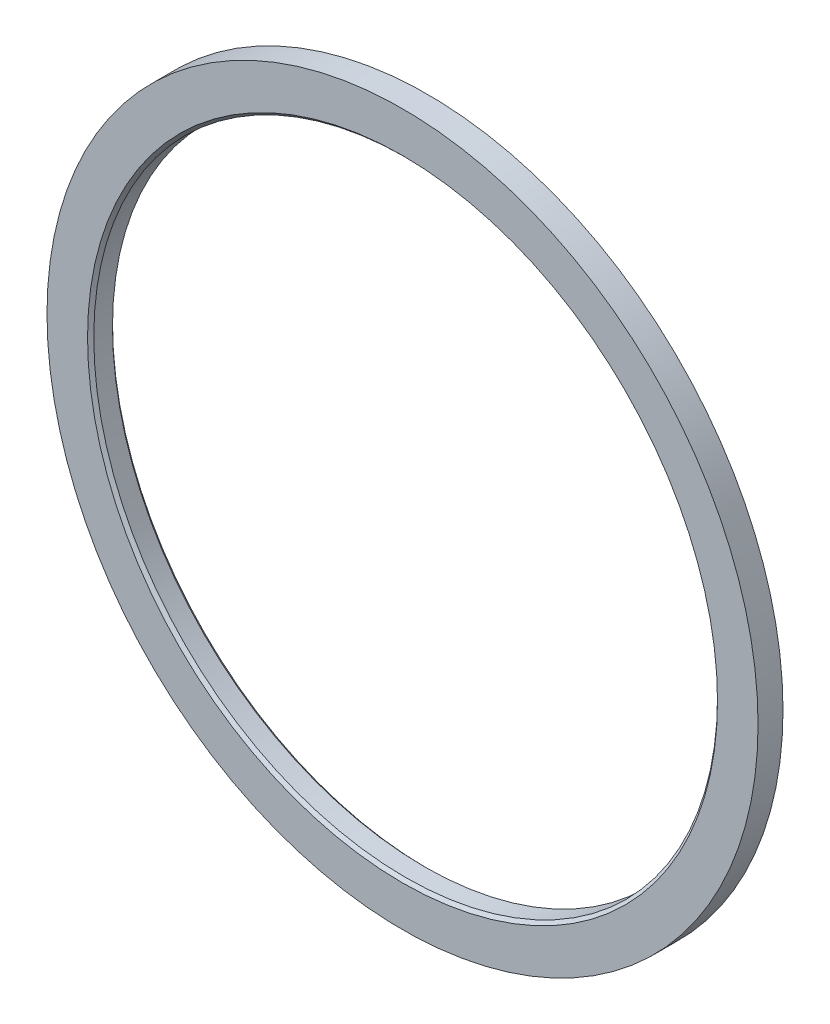
from build123d import *


with BuildPart() as part:
    # Sketch1 → Revolve1 (revolve)
    with BuildSketch(Plane(origin=(0, 234.743963655, 0), x_dir=(1, 0, 0), z_dir=(0, 1, 0))):
        Polygon((571.230642584, 185.192981355), (571.730642584, 184.692981355), (578.230642584, 184.692981355), (578.230642584, 188.692981355), (571.730642584, 188.692981355), (571.230642584, 188.192981355), align=None)
    revolve(axis=Axis((521.230642584, 234.743963655, -188.692981355), (0, 0, 1)))


solid = part.part
